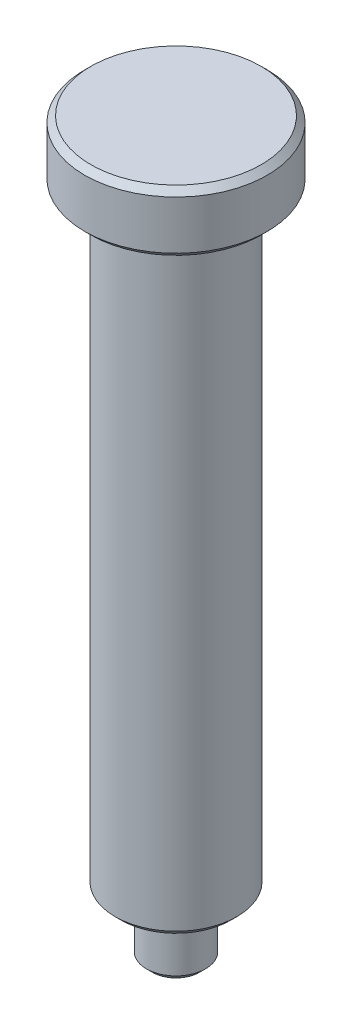
from build123d import *

# Parameters (mm, degrees)
CHAMFER1_SIZE = 0.5


with BuildPart() as part:
    # Sketch1 → Revolve1 (revolve)
    with BuildSketch(Plane(origin=(0, 0, 0), x_dir=(0, 0, -1), z_dir=(1, 0, 0)), mode=Mode.PRIVATE) as revolve1_sk:
        Polygon((0, 0), (7.5, 0), (7.5, -5), (5, -5), (5, -55), (2.425, -55), (2.425, -60), (0, -60), align=None)
    revolve(revolve1_sk.sketch.rotate(Axis((0, 0, 0), (0, -1, 0)), 180), axis=Axis((0, 0, 0), (0, -1, 0)))

    # Chamfer1
    chamfer1_edges = [part.edges().sort_by_distance(p)[0] for p in [
        (0, -60, -2.425),
        (0, -55, -5),
        (0, -5, -7.5),
        (0, 0, -7.5),
    ]]
    chamfer(chamfer1_edges, length=CHAMFER1_SIZE)


solid = part.part
